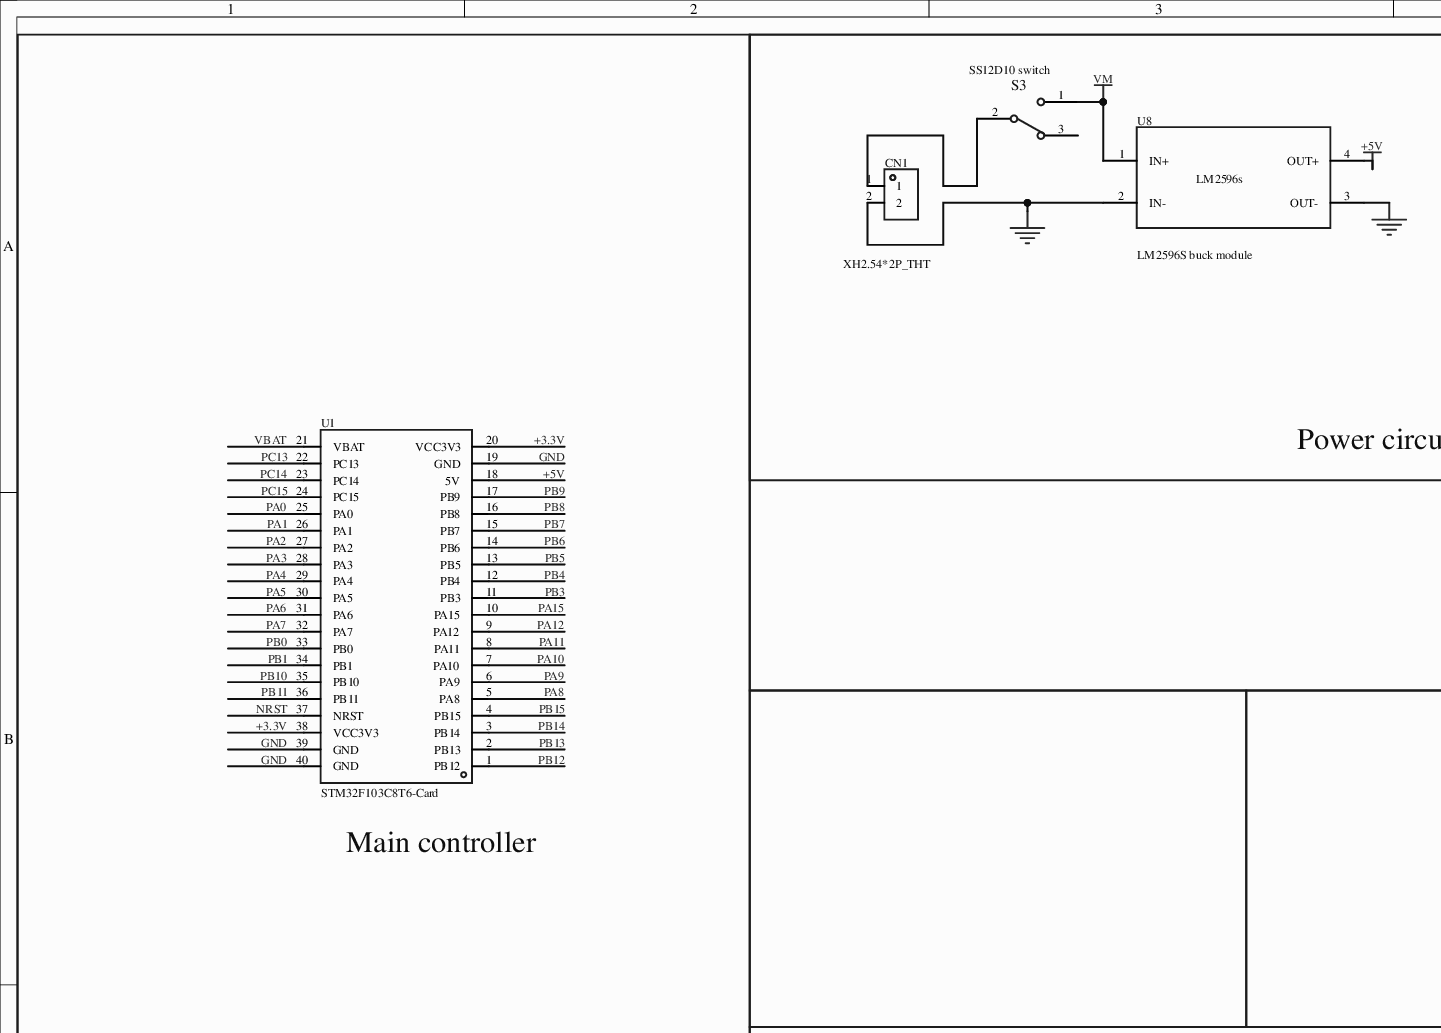
[diagram p0: MISC49897-3.schdoc, top left]
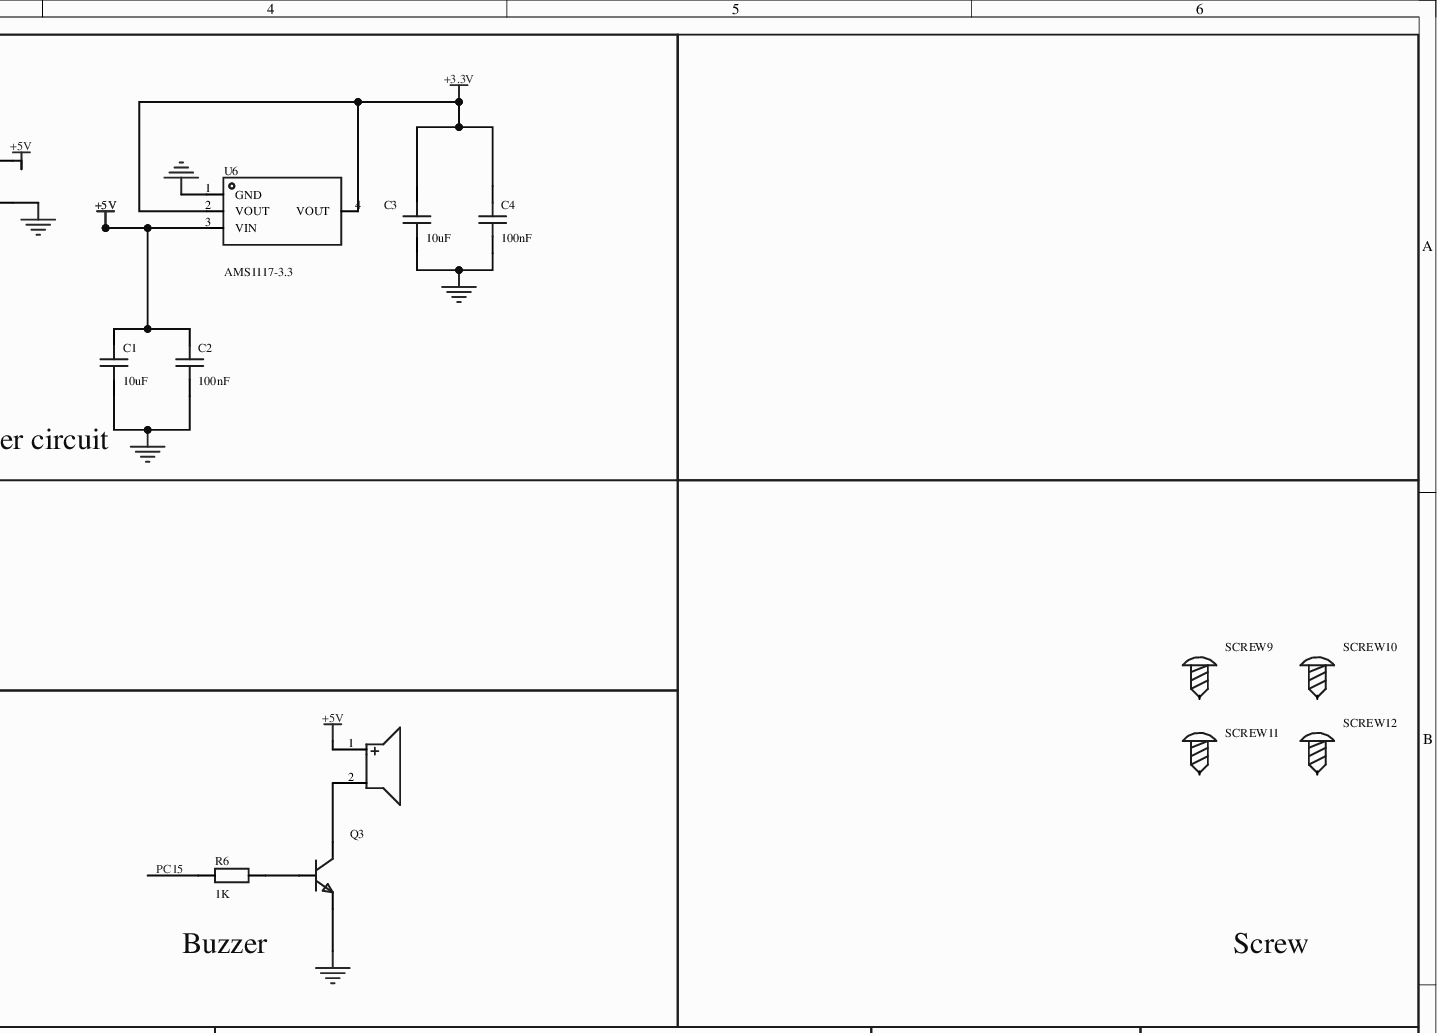
[diagram p1: MISC49897-3.schdoc, top right]
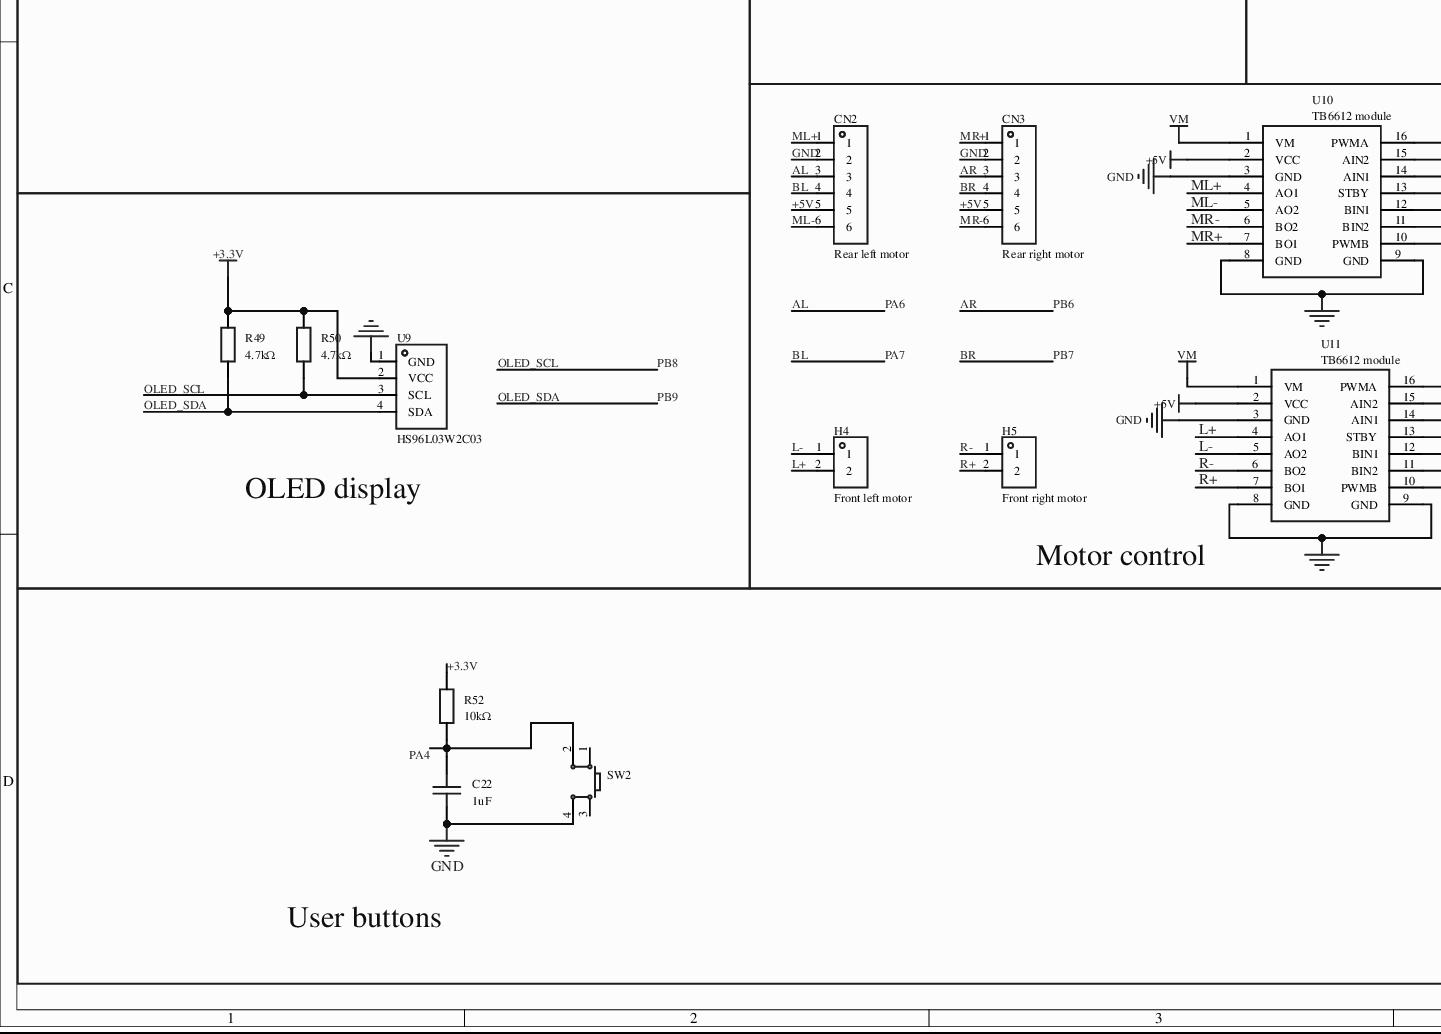
[diagram p2: MISC49897-3.schdoc, bottom left]
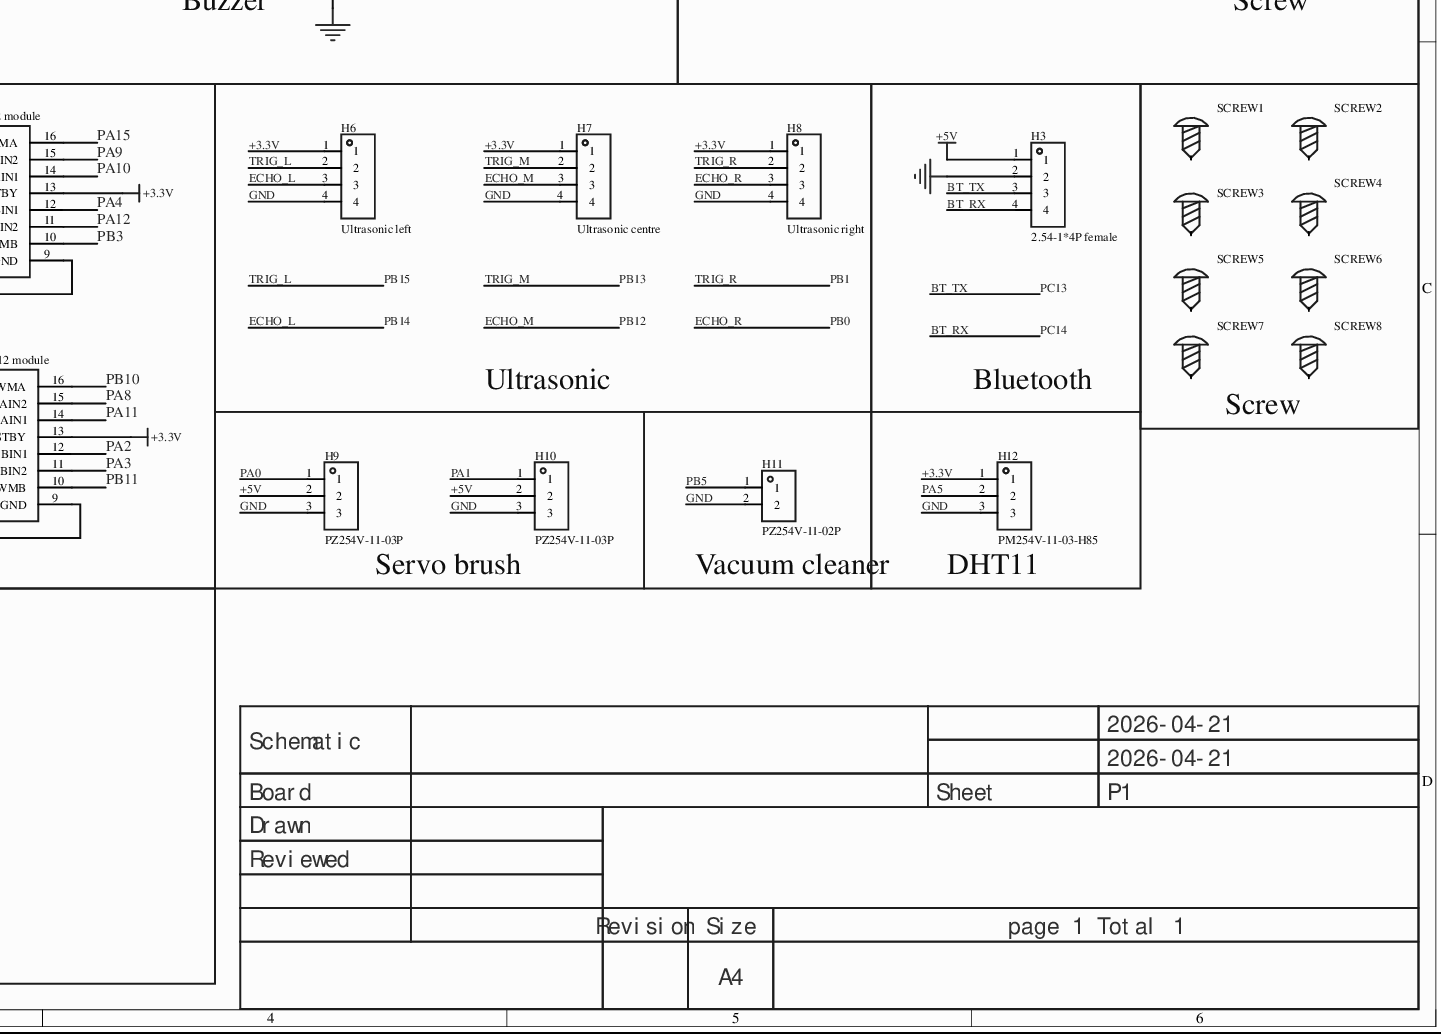
[diagram p3: MISC49897-3.schdoc, bottom right]
# Altium project MISC49897-2.PrjPcb
1 sheet, 44 parts. Net scope: global (net labels, ports and power ports of the same name join across sheets).
Board file: MISC49897.pcbdoc

## Sheet MISC49897-3.schdoc
size 420 x 297 mm; Version: V1.0; @Project Name: MISC49897; @Page Count: 1; @Update Date: 2026-04-21; @Create Date: 2026-04-21; @Schematic Name: MISC49897; @Page No: 1; @Create Time: 17:18:42; @Update Time: 10:03:47; @Board Name: MISC49897

### Parts
BUZZER1  2.7kHz  [BUZ-TH_BD9.0-P4.00-D0.6-FD]  (value not drawn)
C1  10uF  [C0805]
C2  100nF  [C0805]
C3  10uF  [C0805]
C4  100nF  [C0805]
C22  1uF  [C0603]
CN1  XH2.54*2P_THT  [CONN-TH_2P-P2.50-XH2.54-2P]
CN2  Rear left motor  [CONN-TH_XH2.54-6P]
CN3  Rear right motor  [CONN-TH_XH2.54-6P]
H3  2.54-1*4P female  [HDR-TH_4P-P2.54-V-F]
H4  Front left motor  [HDR-TH_2P-P2.54-V-M]
H5  Front right motor  [HDR-TH_2P-P2.54-V-M]
H6  Ultrasonic left  [HDR-TH_4P-P2.54-V-M]
H7  Ultrasonic centre  [HDR-TH_4P-P2.54-V-M]
H8  Ultrasonic right  [HDR-TH_4P-P2.54-V-M]
H9  PZ254V-11-03P  [HDR-TH_3P-P2.54-V-M]
H10  PZ254V-11-03P  [HDR-TH_3P-P2.54-V-M]
H11  PZ254V-11-02P  [HDR-TH_2P-P2.54-V-M]
H12  PM254V-11-03-H85  [HDR-TH_3P-P2.54-V-F]
Q3  (no value)  [S8050_TO_92]
R6  1K  [Res_1/8W]
R49  4.7kΩ  [R0805]
R50  4.7kΩ  [R0805]
R52  10kΩ  [R0603]
S3  SS12D10 switch  [SS12D10]
SCREW1  (no value)  [M3螺丝]
SCREW2  (no value)  [M3螺丝]
SCREW3  (no value)  [M3螺丝]
SCREW4  (no value)  [M3螺丝]
SCREW5  (no value)  [M2螺丝]
SCREW6  (no value)  [M2螺丝]
SCREW7  (no value)  [M2螺丝]
SCREW8  (no value)  [M2螺丝]
SCREW9  (no value)  [M3螺丝]
SCREW10  (no value)  [M3螺丝]
SCREW11  (no value)  [M3螺丝]
SCREW12  (no value)  [M3螺丝]
SW2  (no value)  [SW-TH_4P-L6.0-W6.0-P4.50-LS6.5]
U1  STM32F103C8T6-Card  [CONN-TH_L53.3-W22.9_STM32F103C8T6-CARD]
U6  AMS1117-3.3  [SOT-223-3_L6.5-W3.4-P2.30-LS7.0-BR]
U8  LM2596S buck module  [LM2596S]
U9  HS96L03W2C03  [OLED-TH_L27.8-W27.2-P2.54_C9900033791]
U10  TB6612 module  [TB6612-2X8]
U11  TB6612 module  [TB6612-2X8]

### Blocks framed on the sheet
Main controller: U1
Power circuit: C1-C4 CN1 S3 U6 U8
Screw: SCREW9-SCREW12
Buzzer: BUZZER1 Q3 R6
Motor control: CN2 CN3 H4 H5 U10 U11
Ultrasonic: H6-H8
Bluetooth: H3
Screw: SCREW1-SCREW8
OLED display: R49 R50 U9
Vacuum cleaner: H11
User buttons: C22 R52 SW2

### Nets
+3.3V: C3.2 C4.2 H6.1 H7.1 H8.1 H12.1 R49.1 R50.1 R52.2 U1.20(VCC3V3) U1.38(VCC3V3) U6.2(VOUT) U6.4(VOUT) U9.2(VCC) U10.13(STBY) U11.13(STBY)
+5V: BUZZER1.1 C1.2 C2.2 CN2.5 CN3.5 H3.1 H9.2 H10.2 U1.18(5V) U6.3(VIN) U8.4(OUT+) U10.2(VCC) U11.2(VCC)
GND: C1.1 C2.1 C3.1 C4.1 C22.1 CN1.2 CN2.2 CN3.2 H3.2 H6.4 H7.4 H8.4 H9.3 H10.3 H11.2 H12.3 Q3.1(E) SW2.4 U1.19(GND) U1.39(GND) U1.40(GND) U6.1(GND) U8.2(IN-) U8.3(OUT-) U9.1(GND) U10.3(GND) U10.8(GND) U10.9(GND) U11.3(GND) U11.8(GND) U11.9(GND)
VM: S3.1 U8.1(IN+) U10.1(VM) U11.1(VM)
AL: CN2.3 U1.31(PA6)  [also labelled PA6]
AR: CN3.3 U1.14(PB6)  [also labelled PB6]
BL: CN2.4 U1.32(PA7)  [also labelled PA7]
BR: CN3.4 U1.15(PB7)  [also labelled PB7]
BT_RX: H3.4 U1.23(PC14)  [also labelled PC14]
BT_TX: H3.3 U1.22(PC13)  [also labelled PC13]
ECHO_L: H6.3 U1.3(PB14)  [also labelled PB14]
ECHO_M: H7.3 U1.1(PB12)  [also labelled PB12]
ECHO_R: H8.3 U1.33(PB0)  [also labelled PB0]
L+: H4.2 U11.4(AO1)
L-: H4.1 U11.5(AO2)
ML+: CN2.1 U10.4(AO1)
ML-: CN2.6 U10.5(AO2)
MR+: CN3.1 U10.7(BO1)
MR-: CN3.6 U10.6(BO2)
NRST: U1.37(NRST)
OLED_SCL: R50.2 U1.16(PB8) U9.3(SCL)  [also labelled PB8]
OLED_SDA: R49.2 U1.17(PB9) U9.4(SDA)  [also labelled PB9]
PA0: H9.1 U1.25(PA0)
PA1: H10.1 U1.26(PA1)
PA2: U1.27(PA2) U11.12(BIN1)
PA3: U1.28(PA3) U11.11(BIN2)
PA4: C22.2 R52.1 SW2.2 U1.29(PA4) U10.12(BIN1)
PA5: H12.2 U1.30(PA5)
PA8: U1.5(PA8) U11.15(AIN2)
PA9: U1.6(PA9) U10.15(AIN2)
PA10: U1.7(PA10) U10.14(AIN1)
PA11: U1.8(PA11) U11.14(AIN1)
PA12: U1.9(PA12) U10.11(BIN2)
PA15: U1.10(PA15) U10.16(PWMA)
PB1: H8.2 U1.34(PB1)  [also labelled TRIG_R]
PB3: U1.11(PB3) U10.10(PWMB)
PB4: U1.12(PB4)
PB5: H11.1 U1.13(PB5)
PB10: U1.35(PB10) U11.16(PWMA)
PB11: U1.36(PB11) U11.10(PWMB)
PB13: H7.2 U1.2(PB13)  [also labelled TRIG_M]
PB15: H6.2 U1.4(PB15)  [also labelled TRIG_L]
PC15: R6.1 U1.24(PC15)
R+: H5.2 U11.7(BO1)
R-: H5.1 U11.6(BO2)
VBAT: U1.21(VBAT)
NetBUZZER1_2: BUZZER1.2 Q3.3(C)
NetCN1_1: CN1.1 S3.2
NetQ3_2: Q3.2(B) R6.2

Not connected (* = marked no-connect by the designer): S3 3*; SCREW1 1*; SCREW2 1*; SCREW3 1*; SCREW4 1*; SCREW5 1*; SCREW6 1*; SCREW7 1*; SCREW8 1*; SCREW9 1*; SCREW10 1*; SCREW11 1*; SCREW12 1*; SW2 1 3

### Notes on the sheet
- (near H10) Servo brush
- (near H12) DHT11
- 2026-04-21
- Schematic
- Board
- Sheet
- P1
- Drawn
- Reviewed
- Revision
- Size
- A4
- page 1 Total 1

### Library data of the parts
BUZZER1 = QMB-09B-03: Drive: Passive (external drive); Construction: Electromagnetic; Frequency: 2.7kHz; Sound pressure (SPL): 85dB;; Manufacturer: 华能; 3D Model: 949096c5110a440bbcfd89e7e6948986; 3D Model Transform: 354.33,354.33,0,90,0,0,0,0,-177.165; Voltage - Supply: 2V~5V; AddInBom: yes; ModelName: BUZ-TH_D9.0-H5.5-P4.0; Symbol: QMB-09B-03; Device: QMB-09B-03; LCSC Part Name: 无源蜂鸣器QMB-09B-03; Supplier Part: C96256; Manufacturer Part: QMB-09B-03; Supplier Footprint: 插件,D=9mm; JLCPCB Part Class: Extended library; Datasheet: example.com/upload/public/pdf/source/20210401/C96256_958B17753B5AD7CBFBCFFC7C095B4484.pdf; Supplier: LCSC; Driver Circuitry: Passive (external drive); Technology: Electromagnetic; Value: 2.7kHz; Sound Pressure Level(SPL): 85dB; Diameter(φD): 9mm; Height: 5.7mm; ConvertToPcb: yes; FootprintName: BUZ-TH_BD9.0-P4.00-D0.6-FD
C1 C3 = GRM21BR61H106KE43L: Capacitance: 10uF; Tolerance: ±10%; Rated voltage: 50V; Dielectric (temp. coefficient): X5R;; Manufacturer: muRata(村田); AddInBom: yes; ModelId: 1ba041120af144c991958decab20d241; ModelName: C0805_L2.0-W1.3-H1.3; ModelTransform: 78.74,51.181,0,0,0,0,0,0.0005,0; Symbol: CapAcitance; Device: GRM21BR61H106KE43L; LCSC Part Name: 10uF ±10% 50V; SupplierPart: C440198; ManufacturerPart: GRM21BR61H106KE43L; Supplier Footprint: 0805; JLCPCB Part Class: Basic Part; Datasheet: example.com/upload/public/pdf/source/20230811/95AAE0C9AF55EDC31B7A4D8B733F534E.pdf; Supplier: LCSC; ConvertToPcb: yes; FootprintName: C0805; Value: 10uF; Voltage Rated: 50V; Temperature Coefficient: X5R
C2 C4 = CL21B104KBCNNNC: Capacitance: 100nF; Tolerance: ±10%; Rated voltage: 50V; Dielectric (temp. coefficient): X7R;; Manufacturer: SAMSUNG(三星); AddInBom: yes; ModelId: 1ba041120af144c991958decab20d241; ModelName: C0805_L2.0-W1.3-H1.3; ModelTransform: 78.74,51.181,0,0,0,0,0,0.0005,0; Symbol: CapAcitance; Device: CL21B104KBCNNNC; LCSC Part Name: 100nF ±10% 50V; SupplierPart: C1711; ManufacturerPart: CL21B104KBCNNNC; Supplier Footprint: 0805; JLCPCB Part Class: Extended Part; Datasheet: example.com/upload/public/pdf/source/20160218/1457707763339.pdf; Supplier: LCSC; ConvertToPcb: yes; FootprintName: C0805; Value: 100nF; Voltage Rated: 50V; Temperature Coefficient: X7R
C22 = CL10A105KB8NNNC: Capacitance: 1uF; Tolerance: ±10%; Rated voltage: 50V; Dielectric (temp. coefficient): X5R;; Manufacturer: SAMSUNG(三星); Check: true; AddInBom: yes; ModelId: ac125912035d415993ca9572d50418b1; ModelName: C0603_L1.6-W0.8-H0.8; ModelTransform: 62.992,31.496,0,0,0,0,0,0,0; Symbol: CapAcitance; Device: CL10A105KB8NNNC; Supplier Part: C15849; LCSC Part Name: 1uF ±10% 50V; ManufacturerPart: CL10A105KB8NNNC; Supplier Footprint: 0603; JLCPCB Part Class: Basic Part; Datasheet: example.com/upload/public/pdf/source/20160103/1457707679084.pdf; Supplier: LCSC; ConvertToPcb: yes; FootprintName: C0603; Value: 1uF; Voltage Rated: 50V; Temperature Coefficient: X5R
CN1 = XH2.54*2P_直插: Manufacturer: null; Convert to PCB: yes; ModelId: 325c595e30db4df8abe76612dd40b0fa; Origin Footprint: CONN-TH_2P-P2.50-XH2.54-2P; Device: XH2.54*2P_THT; Symbol: XH2.54*2P_THT; Supplier: LCSC; Supplier Part: C9900008615; Manufacturer Part: XH2.54*2P_直插; JLCPCB Part Class: Extended Part; Add into BOM: yes; FootprintName: CONN-TH_2P-P2.50-XH2.54-2P; link: example.com/pdf/applyPasteComponent/2021-09-13/837084A/aaafcbedaa1341f78bdd46f8ab13ab21/XH2_54datasheet.pdf; 3DModel: CONN-TH_2P-P2.50-XH2.54-2P; ModelName: CONN-TH_2P-P2.50-XH2.54-2P
CN2 = XH2.54*6P_直插: Manufacturer Part: 后左电机; Symbol: XH2.54*6P_THT; AddInBom: yes; ModelId: a7224aacb0dc4305a7392217f7fd8fe2; ModelTransform: 688.975,224.409,0,0,0,0,-0.001,-17.719,-118.11; Device: XH2.54*6P_THT; LCSC Part Name: XH2.54*6P_直插; SupplierPart: C9900008614; Supplier Footprint: XH2.54_6P; JLCPCB Part Class: Extended library; Supplier: LCSC; ConvertToPcb: yes; FootprintName: CONN-TH_XH2.54-6P; ModelName: CONN-TH_XH2.54-6P
CN3 = XH2.54*6P_直插: Manufacturer Part: 后右电机; Symbol: XH2.54*6P_THT; AddInBom: yes; ModelId: a7224aacb0dc4305a7392217f7fd8fe2; ModelTransform: 688.975,224.409,0,0,0,0,-0.001,-17.719,-118.11; Device: XH2.54*6P_THT; LCSC Part Name: XH2.54*6P_直插; SupplierPart: C9900008614; Supplier Footprint: XH2.54_6P; JLCPCB Part Class: Extended library; Supplier: LCSC; ConvertToPcb: yes; FootprintName: CONN-TH_XH2.54-6P; ModelName: CONN-TH_XH2.54-6P
H3 = 2.54-1*4P母: Socket structure: 1x4P; Pitch: 2.54mm; Row spacing: -; Round/square hole: Square hole; Mounting: THT; Rows: Single row; Total holes: 4P; Rated current: 3A; Rated voltage: -; Socket direction: Top; Body height: -; Contact material: Bronze; Contact plating: -; Operating temp. range: -40℃~+105℃; Soldering temp. (max): -;; Manufacturer: BOOMELE(博穆精密); AddInBom: yes; ModelId: d187812051054f85879fcaa51a310d8e; ModelTransform: 419.6842,98.464,0,0,0,0,0,0,-118.11; Symbol: 2.54-1*4P female; Device: 2.54-1*4P female; LCSC Part Name: 间距:2.54mm 1x4P 直插; SupplierPart: C2718488; ManufacturerPart: 2.54-1*4P母; Supplier Footprint: 插件,P=2.54mm; JLCPCB Part Class: Extended library; Datasheet: example.com/upload/public/pdf/source/20210301/C2718488_F4427B881E42CAA8DDB0B1C12B3A522C.pdf; Supplier: LCSC; ConvertToPcb: yes; FootprintName: HDR-TH_4P-P2.54-V-F; ModelName: HDR-TH_4P-P2.54-V-F; Holes Structure: 1x4P; Row Spacing: -; Circular Hole / Square Hole: Square hole; Mounting Type: THT; Number of Rows: Single row; Number of Holes: 4P; Current Rating (Max): 3A; Voltage Rating (Max): -; Holes Direction: Top; Insulation Height: -; Contact Material: Bronze; Contact Plating: -; Operating Temperature Range: -40℃~+105℃; Soldering Temperature(Max): -
H4 = PZ254V-11-02P: Pin structure: 1x2P; Pitch: 2.54mm; Row spacing: -; Round/square pin: Square pin; Mounting: THT; Rows: Single row; Total pins: 2P; Rated current: -; Rated voltage: -; Mating pin length: 6mm; Body height: 2.5mm; Tail length: 3mm; Contact material: Brass; Contact plating: -; Operating temp.: -40℃~+105℃; Color: Black;; Manufacturer Part: 前左电机; Manufacturer: XFCN(兴飞); AddInBom: yes; ModelId: e35305ec3aa84b66b849f914b715e73f; ModelName: HDR2.54-M-LI-1X2P; ModelTransform: 200,100,0,0,0,0,0,0,-118.11; Symbol: PZ254V-11-02P; Device: PZ254V-11-02P; LCSC Part Name: 1x2P 间距:2.54mm 方针 直插; SupplierPart: C492401; Supplier Footprint: 插件,P=2.54mm; JLCPCB Part Class: Extended library; Datasheet: example.com/upload/public/pdf/source/20200309/C492401_A812433581A9B211A7FFA413ADDFF0E5.pdf; Supplier: LCSC; ConvertToPcb: yes; FootprintName: HDR-TH_2P-P2.54-V-M; Pin Structure: 1x2P; Row Spacing: -; Circluar Pins/Square Pins: Square pin; Mounting Type: THT; Number of Rows: Single row; Number of Pins: 2P; Current Rating: -; Voltage Rating (Max): -; Length of Mating Pin: 6mm; Insulation Height: 2.5mm; Length of End Connection Pin: 3mm; Contact Material: Brass; Contact Plating: -; Operating Temperature: -40℃~+105℃; Color: Black
H5 = PZ254V-11-02P: Pin structure: 1x2P; Pitch: 2.54mm; Row spacing: -; Round/square pin: Square pin; Mounting: THT; Rows: Single row; Total pins: 2P; Rated current: -; Rated voltage: -; Mating pin length: 6mm; Body height: 2.5mm; Tail length: 3mm; Contact material: Brass; Contact plating: -; Operating temp.: -40℃~+105℃; Color: Black;; Manufacturer Part: 前右电机; Manufacturer: XFCN(兴飞); AddInBom: yes; ModelId: e35305ec3aa84b66b849f914b715e73f; ModelName: HDR2.54-M-LI-1X2P; ModelTransform: 200,100,0,0,0,0,0,0,-118.11; Symbol: PZ254V-11-02P; Device: PZ254V-11-02P; LCSC Part Name: 1x2P 间距:2.54mm 方针 直插; SupplierPart: C492401; Supplier Footprint: 插件,P=2.54mm; JLCPCB Part Class: Extended library; Datasheet: example.com/upload/public/pdf/source/20200309/C492401_A812433581A9B211A7FFA413ADDFF0E5.pdf; Supplier: LCSC; ConvertToPcb: yes; FootprintName: HDR-TH_2P-P2.54-V-M; Pin Structure: 1x2P; Row Spacing: -; Circluar Pins/Square Pins: Square pin; Mounting Type: THT; Number of Rows: Single row; Number of Pins: 2P; Current Rating: -; Voltage Rating (Max): -; Length of Mating Pin: 6mm; Insulation Height: 2.5mm; Length of End Connection Pin: 3mm; Contact Material: Brass; Contact Plating: -; Operating Temperature: -40℃~+105℃; Color: Black
H6 = PZ254V-11-04P: Pin structure: 1x4P; Pitch: 2.54mm; Row spacing: -; Round/square pin: Square pin; Mounting: THT; Rows: Single row; Total pins: 4P; Rated current: 3A; Rated voltage: 250V; Mating pin length: 6mm; Body height: 2.5mm; Tail length: 3mm; Contact material: -; Operating temp. range: -40℃~+105℃; Color: Black;; Manufacturer Part: 超声波左; Manufacturer: XFCN(兴飞); Symbol: PZ254V-11-04P_C2691448; AddInBom: yes; ModelId: 112f4d05e8d64e99ab9a333894bea4f9; ModelName: HDR-TH_4P-P2.54-M-LI-1X4P; ModelTransform: 399.999,104.7242,0,0,0,0,0,0,-118.11; Device: PZ254V-11-04P; LCSC Part Name: 间距:2.54mm 1x4P 直插 方针; SupplierPart: C2691448; Supplier Footprint: 插件,P=2.54mm; JLCPCB Part Class: Extended library; Datasheet: example.com/upload/public/pdf/source/20200309/C492403_F9F19131791D08044AD4F84F8E751A34.pdf; Supplier: LCSC; ConvertToPcb: yes; FootprintName: HDR-TH_4P-P2.54-V-M; Pin Structure: 1x4P; Row Spacing: -; Circluar Pins/Square Pins: Square pin; Mounting Type: THT; Number of Rows: Single row; Number of Pins: 4P; Current Rating (Max): 3A; Voltage Rating (Max): 250V; Length of Mating Pin: 6mm; Insulation Height: 2.5mm; Length of End Connection Pin: 3mm; Contact Material: -; Operating Temperature Range: -40℃~+105℃; Color: Black
H7 = PZ254V-11-04P: Pin structure: 1x4P; Pitch: 2.54mm; Row spacing: -; Round/square pin: Square pin; Mounting: THT; Rows: Single row; Total pins: 4P; Rated current: 3A; Rated voltage: 250V; Mating pin length: 6mm; Body height: 2.5mm; Tail length: 3mm; Contact material: -; Operating temp. range: -40℃~+105℃; Color: Black;; Manufacturer Part: 超声波中; Manufacturer: XFCN(兴飞); Symbol: PZ254V-11-04P_C2691448; AddInBom: yes; ModelId: 112f4d05e8d64e99ab9a333894bea4f9; ModelName: HDR-TH_4P-P2.54-M-LI-1X4P; ModelTransform: 399.999,104.7242,0,0,0,0,0,0,-118.11; Device: PZ254V-11-04P; LCSC Part Name: 间距:2.54mm 1x4P 直插 方针; SupplierPart: C2691448; Supplier Footprint: 插件,P=2.54mm; JLCPCB Part Class: Extended library; Datasheet: example.com/upload/public/pdf/source/20200309/C492403_F9F19131791D08044AD4F84F8E751A34.pdf; Supplier: LCSC; ConvertToPcb: yes; FootprintName: HDR-TH_4P-P2.54-V-M; Pin Structure: 1x4P; Row Spacing: -; Circluar Pins/Square Pins: Square pin; Mounting Type: THT; Number of Rows: Single row; Number of Pins: 4P; Current Rating (Max): 3A; Voltage Rating (Max): 250V; Length of Mating Pin: 6mm; Insulation Height: 2.5mm; Length of End Connection Pin: 3mm; Contact Material: -; Operating Temperature Range: -40℃~+105℃; Color: Black
H8 = PZ254V-11-04P: Pin structure: 1x4P; Pitch: 2.54mm; Row spacing: -; Round/square pin: Square pin; Mounting: THT; Rows: Single row; Total pins: 4P; Rated current: 3A; Rated voltage: 250V; Mating pin length: 6mm; Body height: 2.5mm; Tail length: 3mm; Contact material: -; Operating temp. range: -40℃~+105℃; Color: Black;; Manufacturer Part: 超声波右; Manufacturer: XFCN(兴飞); Symbol: PZ254V-11-04P_C2691448; AddInBom: yes; ModelId: 112f4d05e8d64e99ab9a333894bea4f9; ModelName: HDR-TH_4P-P2.54-M-LI-1X4P; ModelTransform: 399.999,104.7242,0,0,0,0,0,0,-118.11; Device: PZ254V-11-04P; LCSC Part Name: 间距:2.54mm 1x4P 直插 方针; SupplierPart: C2691448; Supplier Footprint: 插件,P=2.54mm; JLCPCB Part Class: Extended library; Datasheet: example.com/upload/public/pdf/source/20200309/C492403_F9F19131791D08044AD4F84F8E751A34.pdf; Supplier: LCSC; ConvertToPcb: yes; FootprintName: HDR-TH_4P-P2.54-V-M; Pin Structure: 1x4P; Row Spacing: -; Circluar Pins/Square Pins: Square pin; Mounting Type: THT; Number of Rows: Single row; Number of Pins: 4P; Current Rating (Max): 3A; Voltage Rating (Max): 250V; Length of Mating Pin: 6mm; Insulation Height: 2.5mm; Length of End Connection Pin: 3mm; Contact Material: -; Operating Temperature Range: -40℃~+105℃; Color: Black
H9 H10 = PZ254V-11-03P: Pin structure: 1x3P; Pitch: 2.54mm; Row spacing: -; Round/square pin: Square pin; Mounting: THT; Rows: Single row; Total pins: 3P; Rated current: 3A; Rated voltage: 250V; Mating pin length: 6mm; Body height: 2.5mm; Tail length: 3mm; Operating temp.: -40℃~+105℃; Color: Black;; Manufacturer: XFCN(兴飞); Symbol: PZ254V-11-03P_C2937625; AddInBom: yes; ModelId: bb473b6d38ff42a99216a4fcdbdcc4cb; ModelName: HDR-TH_3P-P2.54-M-LI-1X3P; ModelTransform: 299.9994,100,0,0,0,0,0,0,-118.11; Device: PZ254V-11-03P; LCSC Part Name: 1x3P 间距:2.54mm 方针 直插; SupplierPart: C2937625; ManufacturerPart: PZ254V-11-03P; Supplier Footprint: 插件,P=2.54mm; JLCPCB Part Class: Extended library; Datasheet: example.com/upload/public/pdf/source/20200309/C492402_8335C3D49C4E4C618838D59BB1D024C1.pdf; Supplier: LCSC; ConvertToPcb: yes; FootprintName: HDR-TH_3P-P2.54-V-M; Pin Structure: 1x3P; Row Spacing: -; Circluar Pins/Square Pins: Square pin; Mounting Type: THT; Number of Rows: Single row; Number of Pins: 3P; Current Rating: 3A; Voltage Rating (Max): 250V; Length of Mating Pin: 6mm; Insulation Height: 2.5mm; Length of End Connection Pin: 3mm; Operating Temperature: -40℃~+105℃; Color: Black
H11 = PZ254V-11-02P: Pin structure: 1x2P; Pitch: 2.54mm; Row spacing: -; Round/square pin: Square pin; Mounting: THT; Rows: Single row; Total pins: 2P; Rated current: -; Rated voltage: -; Mating pin length: 6mm; Body height: 2.5mm; Tail length: 3mm; Contact material: Brass; Contact plating: -; Operating temp.: -40℃~+105℃; Color: Black;; Manufacturer: XFCN(兴飞); AddInBom: yes; ModelId: e35305ec3aa84b66b849f914b715e73f; ModelName: HDR2.54-M-LI-1X2P; ModelTransform: 200,100,0,0,0,0,0,0,-118.11; Symbol: PZ254V-11-02P; Device: PZ254V-11-02P; LCSC Part Name: 1x2P 间距:2.54mm 方针 直插; SupplierPart: C492401; ManufacturerPart: PZ254V-11-02P; Supplier Footprint: 插件,P=2.54mm; JLCPCB Part Class: Extended library; Datasheet: example.com/upload/public/pdf/source/20200309/C492401_A812433581A9B211A7FFA413ADDFF0E5.pdf; Supplier: LCSC; ConvertToPcb: yes; FootprintName: HDR-TH_2P-P2.54-V-M; Pin Structure: 1x2P; Row Spacing: -; Circluar Pins/Square Pins: Square pin; Mounting Type: THT; Number of Rows: Single row; Number of Pins: 2P; Current Rating: -; Voltage Rating (Max): -; Length of Mating Pin: 6mm; Insulation Height: 2.5mm; Length of End Connection Pin: 3mm; Contact Material: Brass; Contact Plating: -; Operating Temperature: -40℃~+105℃; Color: Black
H12 = PM254V-11-03-H85: Socket structure: 1x3P; Pitch: 2.54mm; Row spacing: -; Mounting: THT; Rows: Single row; Total holes: 3P; Body height: -; Contact material: Brass; Contact plating: -;; Manufacturer: XFCN(兴飞); AddInBom: yes; ModelId: f3b3cc5aae9641bf9e56fc160cef875b; ModelName: HDR2.54-F-LI-1X3P; ModelTransform: 299.9994,100,0,0,0,0,0,0,-118.11; Symbol: PM254V-11-03-H85; Device: PM254V-11-03-H85; LCSC Part Name: 间距:2.54mm 1x3P 直插; SupplierPart: C541850; ManufacturerPart: PM254V-11-03-H85; Supplier Footprint: 插件,P=2.54mm; JLCPCB Part Class: Extended library; Datasheet: example.com/upload/public/pdf/source/20200518/C541849_85853D71FC67C51915A806977A588FDA.pdf; Supplier: LCSC; ConvertToPcb: yes; FootprintName: HDR-TH_3P-P2.54-V-F; Holes Structure: 1x3P; Row Spacing: -; Mounting Type: THT; Number of Rows: Single row; Number of Holes: 3P; Insulation Height: -; Contact Material: Brass; Contact Plating: -
Q3 = S8050_TO_NPN: 3D Model: aafe8e06f2154e7c93506efd0d6632dd; 3D Model Transform: 180.78,141.44,417.3,0,0,0,0,0,-200; ConvertToPcb: yes; ModelName: TO-92-3_L4.9-W3.7-P1.27-L; Symbol: S8050_TO_NPN; Device: S8050_TO_NPN; Supplier Footprint: TO-92; AddInBom: yes; FootprintName: S8050_TO_92
R6 = Res_AXIAL-1/8W: Symbol: Resistor; 3D Model: b2b5ae7ae4c642178fe0039925c86a3f; 3D Model Transform: 282.86,66.88,253.09,0,0,0,0,0,-191; ConvertToPcb: yes; ModelName: RES-TH_BD1.8-L3.2-P7.20-D0.4; Device: Res_AXIAL-1/8W; Value: 1K; Supplier Footprint: 轴向引线; AddInBom: yes; FootprintName: Res_1/8W
R49 R50 = 0805W8F4701T5E: Resistor type: Thick-film resistor; Resistance: 4.7kΩ; Tolerance: ±1%; Power: 125mW; Max working voltage: 150V; Temp. coefficient: ±100ppm/℃;; Manufacturer: UNI-ROYAL(厚声); AddInBom: yes; ModelId: 37a81e68749a4138bd2dfa6897b24b85; ModelName: R0805_L2.0-W1.3-H0.6; ModelTransform: 78.74,51.181,0,0,0,0,0,-0.0005,0; Symbol: 0805W8F4701T5E; Device: 0805W8F4701T5E; LCSC Part Name: 4.7kΩ ±1% 125mW 厚膜电阻; SupplierPart: C17673; ManufacturerPart: 0805W8F4701T5E; Supplier Footprint: 0805; JLCPCB Part Class: Basic library; Datasheet: example.com/upload/public/pdf/source/20200306/C422600_1E6D84923E4A46A82E41ADD87F860B5C.pdf; Supplier: LCSC; ConvertToPcb: yes; FootprintName: R0805; Type: Thick-film resistor; Value: 4.7kΩ; Power(Watts): 125mW; Overload Voltage (Max): 150V; Temperature Coefficient: ±100ppm/℃; Operating Temperature Range: -55℃~+155℃
R52 = 0603WAF1002T5E: Resistor type: Thick-film resistor; Resistance: 10kΩ; Tolerance: ±1%; Power: 100mW;; Manufacturer: UNI-ROYAL(厚声); Check: true; AddInBom: yes; ModelId: fc143cca1e79419f9cd78b61e9279f08; ModelTransform: 31.8897,63.7794,0,90,0,0,0,0,0; Temperature Coefficient: ±100ppm/℃; Overload Voltage (Max): 75V; Symbol: Resistor; Device: 0603WAF1002T5E; LCSC Part Name: 10kΩ ±1% 100mW; SupplierPart: C25804; ManufacturerPart: 0603WAF1002T5E; Supplier Footprint: 0603; JLCPCB Part Class: Basic Part; Datasheet: example.com/upload/public/pdf/source/20200306/C422600_1E6D84923E4A46A82E41ADD87F860B5C.pdf; Supplier: LCSC; ConvertToPcb: yes; FootprintName: R0603; ModelName: R0603; Type: Thick-film resistor; Value: 10kΩ; Power(Watts): 100mW; Operating Temperature Range: -55℃~+155℃
S3 = SS12D10: AddInBom: yes; _: 3; Symbol: SS12D10; Device: SS12D10; ConvertToPcb: yes; FootprintName: SS12D10
SCREW1-SCREW4 = M3螺丝: Device: M3 screw; ConvertToPcb: yes; SymbolName: Screw hole; AddInBom: yes; Supplier Footprint: 插件; FootprintName: M3 screw
SCREW5-SCREW8 = M2螺丝: Device: M2 screw; ConvertToPcb: yes; SymbolName: Screw hole; AddInBom: yes; Supplier Footprint: 插件; FootprintName: M2 screw
SCREW9-SCREW12 = M3螺丝: Symbol: Screw hole; Device: M3 screw; ConvertToPcb: yes; Supplier Footprint: 插件; AddInBom: yes; FootprintName: M3 screw
SW2 = Key_TH_6x6x6: Contact current: 50mA; Rated voltage (DC): 12V; Insulation resistance: 100MΩ; Circuit: SPST; Mounting: THT; Button shape: Round button; Button/cap colour: Black; Actuation force: 260gf@±30gf; Operating temp.: -25℃~+70℃; Pin style: PC pin; Switch length: 6mm; Switch width: 6mm; Switch height: 6mm; With bracket: No;; Symbol: Tactile switch; AddInBom: yes; ModelId: 20eee248bc684ccd8cbdbb1d0d91ec6f0819f05c4eef4c71ace90d822a990e87; ModelName: SW-TH_4P-L6.0-W6.0-H5.0-LS6.5-P4.50; ModelTransform: 236.22,323.03,0,90,0,0,0,0,-137.795; Device: Key_TH_6x6x6; ConvertToPcb: yes; FootprintName: SW-TH_4P-L6.0-W6.0-P4.50-LS6.5; Supplier Footprint: 插件
U1 = STM32F103C8T6-Card: AddInBom: yes; Symbol: STM32F103C8T6-CARD; Device: STM32F103C8T6-Card; LCSC Part Name: STM32F103C8T6-Card; Supplier Part: C9900077949; Manufacturer Part: STM32F103C8T6-Card; Supplier Footprint: 插件; Supplier: LCSC; FootprintName: CONN-TH_L53.3-W22.9_STM32F103C8T6-CARD; ConvertToPcb: yes
U6 = AMS1117-3.3_C6186: Output type: Fixed; Output polarity: Positive; Max input voltage: -; Output voltage: 3.3V; Output current: 1A; PSRR: 72dB@(120Hz);; Manufacturer: AMS; AddInBom: yes; ModelId: 925194bf9823436183a3e0b978a8d076; ModelName: SOT-223-4P_L6.5-W3.5-H1.6-LS7.0-P2.30; ModelTransform: 279.89794,255.905,0,180,0,0,-3.9385,-0.0005,0; Number of Outputs: 1; Dropout Voltage: 1.3V@(800mA); Device: AMS1117-3.3_C6186; Symbol: AMS1117-3.3; LCSC Part Name: 输出3.3V 1A; SupplierPart: C6186; ManufacturerPart: AMS1117-3.3; Supplier Footprint: SOT-223; JLCPCB Part Class: Basic library; Datasheet: example.com/upload/public/pdf/source/20180727/C6186_7A095716F0823C02F1997A905E26C086.pdf; Supplier: LCSC; ConvertToPcb: yes; FootprintName: SOT-223-3_L6.5-W3.4-P2.30-LS7.0-BR; Output Type: Fixed; Output Polarity: Positive; Maximum Input Voltage: -; Output Voltage: 3.3V; Quiescent Current (Ground Current): -; Output Current: 1A; Power Supply Rejection Ratio (PSRR): 72dB@(120Hz); Noise: -; Feature: -; Operating Temperature: -
U8 = LM2596S: Convert to PCB: yes; Symbol: LM2596S; Device: LM2596S; Add into BOM: yes; FootprintName: LM2596S
U9 = HS96L03W2C03: Controller: SSD1315; Interface: I2C; Size (inch): 0.96; Pixel resolution: 128x64;; Manufacturer: HS(汉昇); AddInBom: yes; ModelId: bb65183306db4ca69fb52250be49b00e; ModelTransform: 1070.864,1094.486,0,0,0,0,0,-468.503,0; Symbol: HS96L03W2C03; Device: HS96L03W2C03; LCSC Part Name: 0.96寸OLED显示屏窄白光IIC; SupplierPart: C5248080; ManufacturerPart: HS96L03W2C03; Supplier Footprint: -; JLCPCB Part Class: Extended library; Datasheet: example.com/upload/public/pdf/source/20230627/763D01F79A90007632F098068C7C8AD9.pdf; Supplier: LCSC; ConvertToPcb: yes; FootprintName: OLED-TH_L27.8-W27.2-P2.54_C9900033791; ModelName: OLED-TH_L27.8-W27.2-P2.54_C9900033791; Main Control Chip: SSD1315; Interface Type: I2C; Size: 0.96; Pixel Resolution: 128x64; Operating Temperature: -40℃~+70℃
U10 U11 = TB6612模块: Convert to PCB: yes; Origin Footprint: TB6612-2X8; Device: TB6612 module; Symbol: TB6612 module; Add into BOM: yes; FootprintName: TB6612-2X8